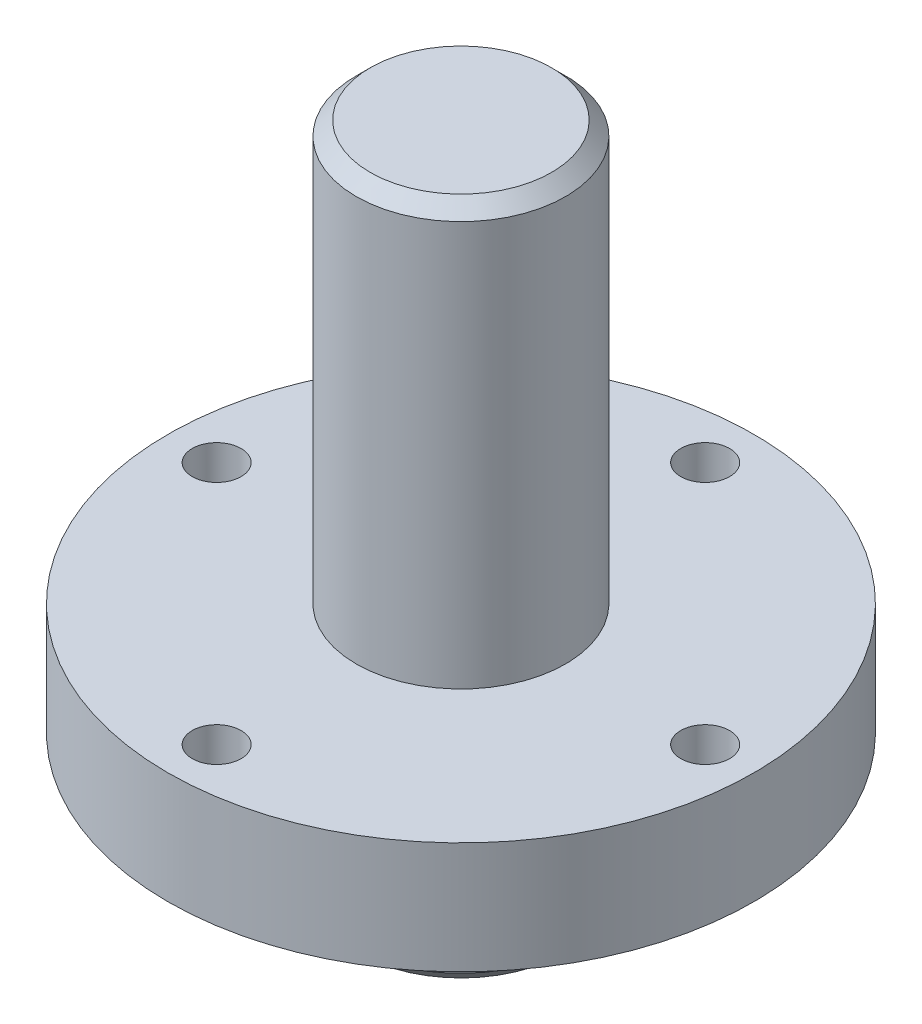
SolidWorks part; units mm, degrees
ref_plane "Front Plane" through (0, 0, 0) normal (0, 0, 1) x (1, 0, 0)
ref_plane "Top Plane" through (0, 0, 0) normal (0, 1, 0) x (1, 0, 0)
ref_plane "Right Plane" through (0, 0, 0) normal (1, 0, 0) x (0, 0, -1)
sketch "Sketch1" plane through (0, 0, 0) normal (0, 1, 0) x (1, 0, 0)
  circle A0 centre (0, 0) radius 15
  dimension "D1" = 30
extrude "Boss-Extrude1" add sketch "Sketch1" along normal blind 65
sketch "Sketch2" plane through (0, 0, 0) normal (0, -1, 0) x (1, 0, 0)
  circle A0 centre (0, 0) radius 14
  dimension "D1" = 28
extrude "Boss-Extrude2" add sketch "Sketch2" along normal blind 260
sketch "Sketch3" plane through (0, -260, 0) normal (0, -1, 0) x (1, 0, 0)
  line L0 (0, 0) -> (50000, 0) construction
  line L1 (0, 0) -> (0, -50000) construction
  line L2 (-11.0039, -13) -> (11.0039, -13)
  line L3 (-11.0039, 15) -> (11.0039, 15)
  line L4 (-11.0039, 15) -> (-11.0039, 13)
  line L5 (-11.0039, 13) -> (11.0039, 13)
  line L6 (11.0039, 15) -> (11.0039, 13)
  line L7 (-11.0039, 15) -> (11.0039, 13) construction
  line L8 (-11.0039, 13) -> (11.0039, 15) construction
  line L9 (11.0039, -15) -> (11.0039, -13)
  line L10 (-11.0039, -15) -> (11.0039, -15)
  line L11 (-11.0039, -15) -> (-11.0039, -13)
  line L12 (-11.0039, -13) -> (11.0039, -15) construction
  line L13 (-11.0039, -15) -> (11.0039, -13) construction
  circle A0 centre (0, 0) radius 14 construction
  point P5 (0, 14)
  point P16 (0, -14)
  dimension "D1" = 26
extrude "Cut-Extrude1" cut sketch "Sketch3" against normal blind 22
pattern_circular "CirPattern1" count 4 every 90 about axis through (0, -260, 0) along (0, 1, 0) of "Cut-Extrude1"
sketch "Sketch4" plane through (0, -260, 0) normal (0, -1, 0) x (1, 0, 0)
  circle A0 centre (0, 0) radius 10.5
  dimension "D1" = 21
extrude "Boss-Extrude3" add sketch "Sketch4" along normal blind 30
sketch "Sketch5" plane through (0, -290, 0) normal (0, -1, 0) x (1, 0, 0)
  circle A0 centre (0, 0) radius 10.3
  dimension "D1" = 20.6
extrude "Boss-Extrude4" add sketch "Sketch5" along normal blind 10
sketch "Sketch6" plane through (0, -300, 0) normal (0, -1, 0) x (1, 0, 0)
  circle A0 centre (0, 0) radius 10.5
  dimension "D1" = 21
extrude "Boss-Extrude5" add sketch "Sketch6" along normal blind 16
chamfer "Chamfer1" distance 8 distance2 1 1 edges at (0, -316, -10.5)
sketch "Sketch8" plane through (0, 65, 0) normal (0, 1, 0) x (1, 0, 0)
  circle A0 centre (0, 0) radius 7.5
  dimension "D1" = 15
extrude "Boss-Extrude6" add sketch "Sketch8" along normal blind 30
sketch "Sketch11" plane through (0, 65, 0) normal (0, 1, 0) x (1, 0, 0)
  circle A0 centre (0, 0) radius 21
  circle A1 centre (0, 0) radius 15 construction
  circle A2 centre (0, 0) radius 15
  dimension "D1" = 42
extrude "Boss-Extrude7" add sketch "Sketch11" against normal blind 8
sketch "Sketch13" plane through (0, -316, 0) normal (0, -1, 0) x (1, 0, 0)
  circle A0 centre (0, 0) radius 19
  dimension "D1" = 38
extrude "Cut-Extrude4" cut sketch "Sketch13" against normal up to surface (373 mm away) up to face at (0, 57, 15)
sketch "Sketch14" plane through (0, 57, 0) normal (0, -1, 0) x (1, 0, 0)
  circle A0 centre (0, 0) radius 8.4
  dimension "D1" = 16.8
extrude "Boss-Extrude8" add sketch "Sketch14" along normal blind 10
chamfer "Chamfer3" distance 1 angle 45 2 edges at (0, 47, -8.4) (0, 95, 7.5)
sketch "Sketch16" plane through (0, 65, 0) normal (0, 1, 0) x (1, 0, 0)
  line L0 (0, 0) -> (0, 50000) construction
  line L1 (0, 0) -> (50000, 0) construction
  circle A0 centre (0, 0) radius 17.5 construction
  circle A1 centre (17.5, 0) radius 1.75
  dimension "D1" = 35
  dimension "D2" = 3.5
extrude "Cut-Extrude5" cut sketch "Sketch16" against normal through all
pattern_circular "CirPattern3" count 4 over 360 about axis through (0, 0, 0) along (0, 1, 0) of "Cut-Extrude5"
